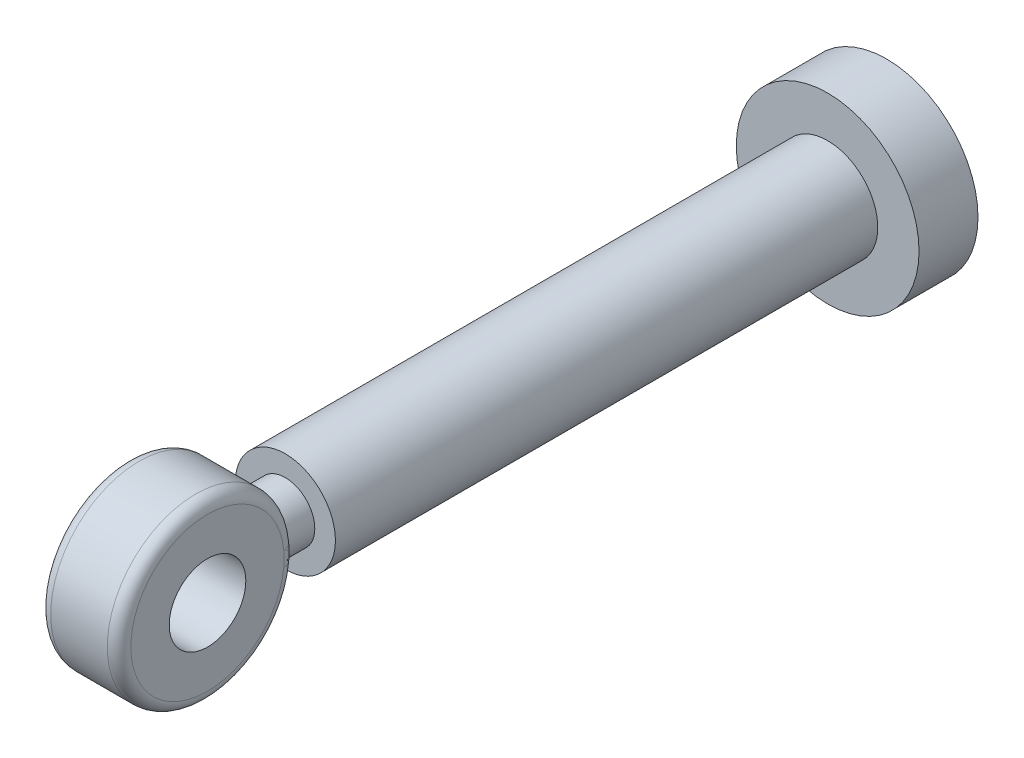
from build123d import *

# Parameters (mm, degrees)
SKETCH_1_R           = 42.5
EXTRUDE_1_DEPTH      = 460
SKETCH_2_R           = 77.5
EXTRUDE_2_DEPTH      = 50
SKETCH_3_R           = 75.00000000000003
SKETCH_3_R_2         = 32.499999999999964
EXTRUDE_3_DEPTH      = 34
EXTRUDE_4_REACH      = 523.644
EXTRUDE_4_END_RADIUS = 75.00000000000003
SKETCH_4_R           = 25
FILLET_1_R           = 10


with BuildPart() as part:
    # 草图1 → 凸台-拉伸1 (new body)
    with BuildSketch(Plane.XY):
        Circle(SKETCH_1_R)
    extrude(amount=EXTRUDE_1_DEPTH)

    # 草图2 → 凸台-拉伸2 (add)
    with BuildSketch(Plane(origin=(0, 0, 0), x_dir=(-1, 0, 0), z_dir=(0, 0, -1))):
        Circle(SKETCH_2_R)
    extrude(amount=EXTRUDE_2_DEPTH)



with BuildPart() as body_2:
    # 草图3 → 凸台-拉伸3 (new, symmetric)
    with BuildSketch(Plane(origin=(0, 0, 0), x_dir=(0, 0, -1), z_dir=(1, 0, 0))):
        with Locations((-560, 0)):
            Circle(SKETCH_3_R)
        with Locations((-560, 0)):
            Circle(SKETCH_3_R_2, mode=Mode.SUBTRACT)
    extrude(amount=EXTRUDE_3_DEPTH, both=True)


with BuildPart() as part_1:
    add(part.part)

    add(body_2.part)  # 凸台-拉伸4 merges body 2
    # 凸台-拉伸4: up to this cylinder (the profile starts outside it)
    extrude_4_end = Plane(origin=(0, 0, 560), z_dir=(-1, 0, 0)) * Cylinder(EXTRUDE_4_END_RADIUS, 1198.288, mode=Mode.PRIVATE)
    # 草图4 → 凸台-拉伸4 (add, up to the surface)
    with BuildSketch(Plane.XY.offset(460), mode=Mode.PRIVATE) as extrude_4_sk1:
        with Locations(Location((0, 0, 0), (0, 0, 180))):
            Circle(SKETCH_4_R)
    extrude_4_tool1 = extrude(extrude_4_sk1.sketch, amount=EXTRUDE_4_REACH, mode=Mode.PRIVATE) - extrude_4_end
    add(extrude_4_tool1.solids().sort_by_distance((0, 0, 460))[0])

    # 圆角1
    fillet_1_edges = [part_1.edges().sort_by_distance(p)[0] for p in [
        (-34, 9.18e-15, 635),
        (34, 9.18e-15, 635),
    ]]
    fillet(fillet_1_edges, radius=FILLET_1_R)


solid = part_1.part
